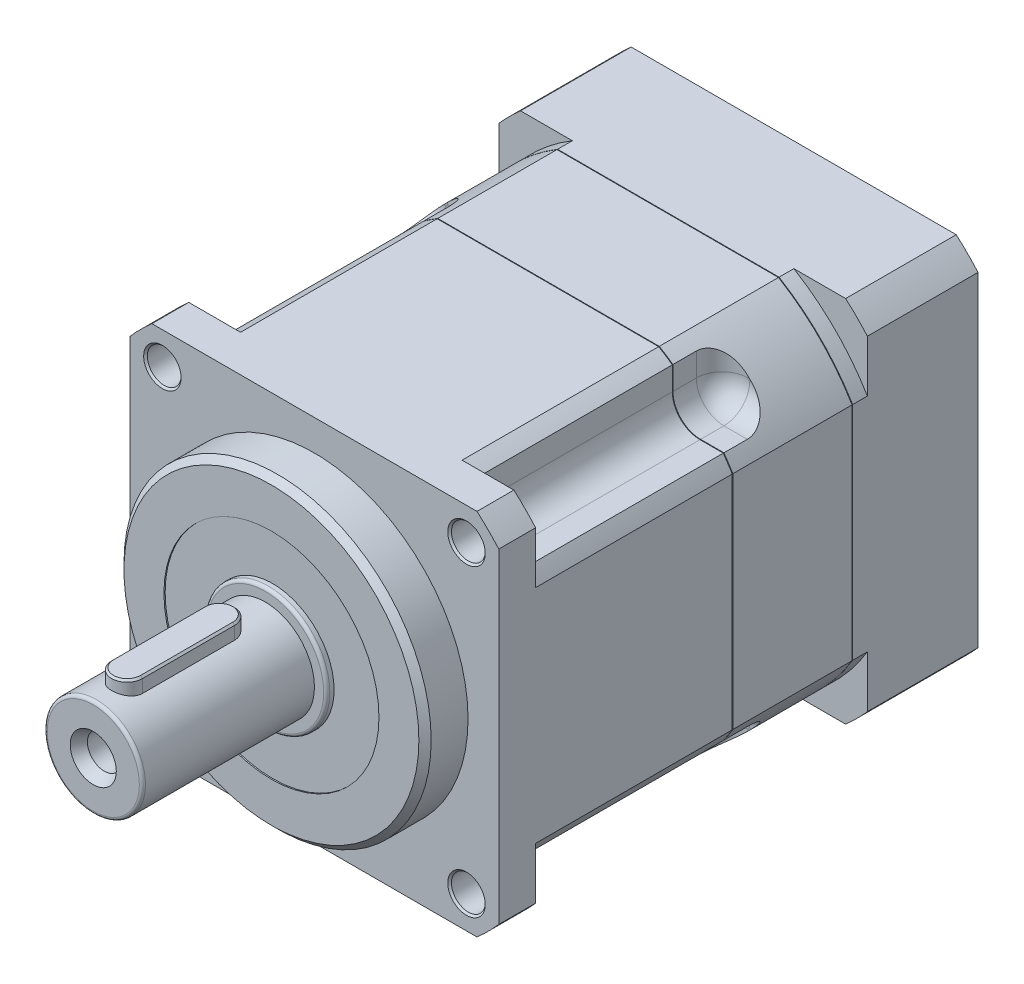
from build123d import *

# Parameters (mm, degrees)
EXTRUDE_1_DEPTH          = 6
SKETCH_2_R               = 25
EXTRUDE_2_DEPTH          = 7
EXTRUDE_3_DEPTH          = 32
SKETCH_4_W               = 13.908632067
SKETCH_4_H               = 13.141259263
CUT_EXTRUDE_1_DEPTH      = 32
PATTERN_CIRCULAR_1_COUNT = 4
FILLET_1_R               = 4.5
SKETCH_5_R               = 2.75
CUT_EXTRUDE_2_DEPTH      = 32
PATTERN_CIRCULAR_2_COUNT = 4
EXTRUDE_4_DEPTH          = 19.4
SKETCH_7_W               = 15.922985677
SKETCH_7_H               = 14.292318469
CUT_EXTRUDE_3_DEPTH      = 8
PATTERN_CIRCULAR_3_COUNT = 4
FILLET_2_R               = 4.5
FILLET_3_R               = 4.2
CHAMFER_1_SIZE           = 1
EXTRUDE_5_DEPTH          = 2.4
EXTRUDE_START            = 18
EXTRUDE_6_DEPTH          = 18
SKETCH_10_R              = 25
CUT_EXTRUDE_4_DEPTH      = 5
SKETCH_11_R              = 4
CUT_EXTRUDE_5_DEPTH      = 12
PATTERN_CIRCULAR_4_COUNT = 4
SKETCH_12_R              = 4
CUT_EXTRUDE_6_DEPTH      = 12
PATTERN_CIRCULAR_5_COUNT = 2
SKETCH_13_R              = 19
CUT_EXTRUDE_7_DEPTH      = 13
SKETCH_14_R              = 3
EXTRUDE_7_DEPTH          = 6
PATTERN_CIRCULAR_6_COUNT = 4
SKETCH_15_R              = 3
EXTRUDE_8_DEPTH          = 6
PATTERN_CIRCULAR_7_COUNT = 2
PATTERN_CIRCULAR_8_COUNT = 4
SKETCH_18_R              = 16.5
EXTRUDE_9_DEPTH          = 11.5
CHAMFER_2_SIZE           = 1
SKETCH_19_R              = 7
CUT_EXTRUDE_8_DEPTH      = 34
SKETCH_20_W              = 35.682835372
SKETCH_20_H              = 1
CUT_EXTRUDE_9_DEPTH      = 11.5
SKETCH_21_R              = 8
EXTRUDE_10_DEPTH         = 29
SKETCH_22_R              = 10
EXTRUDE_11_DEPTH         = 1
FILLET_4_R               = 0.5
FILLET_5_R               = 0.5
CUT_EXTRUDE_START        = -0.2
SKETCH_23_R              = 17.5
SKETCH_23_R_2            = 10
CUT_EXTRUDE_10_DEPTH     = 0.2
EXTRUDE_12_DEPTH         = 10
CHAMFER_3_SIZE           = 0.3
SKETCH_25_R              = 2.75
CUT_EXTRUDE_11_DEPTH     = 4.8
SKETCH_26_R              = 3.75
SKETCH_27_R              = 2.75


with BuildPart() as part:
    # 草图1 → 凸台-拉伸1 (new body)
    with BuildSketch(Plane.XY):
        with BuildLine():
            Line((-26.457513111, 30), (26.457513111, 30))
            ThreePointArc((26.457513111, 30), (28.284271247, 28.284271247), (30, 26.457513111))
            Line((30, 26.457513111), (30, -26.457513111))
            ThreePointArc((30, -26.457513111), (28.284271247, -28.284271247), (26.457513111, -30))
            Line((26.457513111, -30), (-26.457513111, -30))
            ThreePointArc((-26.457513111, -30), (-28.284271247, -28.284271247), (-30, -26.457513111))
            Line((-30, -26.457513111), (-30, 26.457513111))
            ThreePointArc((-30, 26.457513111), (-28.284271247, 28.284271247), (-26.457513111, 30))
        make_face()
    extrude(amount=EXTRUDE_1_DEPTH)

    # 草图2 → 凸台-拉伸2 (add)
    with BuildSketch(Plane.XY.offset(6)):
        Circle(SKETCH_2_R)
    extrude(amount=EXTRUDE_2_DEPTH)

    # 草图3 → 凸台-拉伸3 (add)
    with BuildSketch(Plane(origin=(0, 0, 0), x_dir=(-1, 0, 0), z_dir=(0, 0, -1))):
        with BuildLine():
            Line((-18.027756377, 30), (18.027756377, 30))
            ThreePointArc((18.027756377, 30), (24.748737342, 24.748737342), (30, 18.027756377))
            Line((30, 18.027756377), (30, -18.027756377))
            ThreePointArc((30, -18.027756377), (24.748737342, -24.748737342), (18.027756377, -30))
            Line((18.027756377, -30), (-18.027756377, -30))
            ThreePointArc((-18.027756377, -30), (-24.748737342, -24.748737342), (-30, -18.027756377))
            Line((-30, -18.027756377), (-30, 18.027756377))
            ThreePointArc((-30, 18.027756377), (-24.748737342, 24.748737342), (-18.027756377, 30))
        make_face()
    extrude(amount=EXTRUDE_3_DEPTH)

    # 草图4 → 切除-拉伸1 (cut)
    with BuildSketch(Plane(origin=(0, 0, -32), x_dir=(-1, 0, 0), z_dir=(0, 0, -1))):
        with Locations((-27.204316033, 26.820629632)):
            Rectangle(SKETCH_4_W, SKETCH_4_H)
    cut_extrude_1 = extrude(amount=-CUT_EXTRUDE_1_DEPTH, mode=Mode.SUBTRACT)

    # 阵列(圆周)1: 切除-拉伸1 ×4 about axis
    pattern_circular_1_axis = Axis((0, 0, 0), (0, 0, 1))
    for i in range(1, PATTERN_CIRCULAR_1_COUNT):
        add(cut_extrude_1.rotate(pattern_circular_1_axis, i * 360 / PATTERN_CIRCULAR_1_COUNT), mode=Mode.SUBTRACT)

    # 圆角1
    fillet_1_edges = [part.edges().sort_by_distance(p)[0] for p in [
        (-20.25, -20.25, -16),
        (20.25, -20.25, -16),
        (20.25, 20.25, -16),
        (-20.25, 20.25, -16),
    ]]
    fillet(fillet_1_edges, radius=FILLET_1_R)

    # 草图5 → 切除-拉伸2 (cut)
    with BuildSketch(Plane.XY.offset(6)):
        with Locations((-24.748737342, 24.748737342)):
            Circle(SKETCH_5_R)
    cut_extrude_2 = extrude(amount=-CUT_EXTRUDE_2_DEPTH, mode=Mode.SUBTRACT)

    # 阵列(圆周)2: 切除-拉伸2 ×4 about axis
    pattern_circular_2_axis = Axis((0, 0, 0), (0, 0, 1))
    for i in range(1, PATTERN_CIRCULAR_2_COUNT):
        add(cut_extrude_2.rotate(pattern_circular_2_axis, i * 360 / PATTERN_CIRCULAR_2_COUNT), mode=Mode.SUBTRACT)

    # 倒角1
    chamfer_1_edges = [part.edges().sort_by_distance(p)[0] for p in [
        (-25, 0, 13),
    ]]
    chamfer(chamfer_1_edges, length=CHAMFER_1_SIZE)

    # 草图21 → 凸台-拉伸10 (add)
    with BuildSketch(Plane.XY.offset(13)):
        with Locations(Location((0, 0, 0), (0, 0, 180))):
            Circle(SKETCH_21_R)
    extrude(amount=EXTRUDE_10_DEPTH)

    # 草图22 → 凸台-拉伸11 (add)
    with BuildSketch(Plane.XY.offset(13)):
        Circle(SKETCH_22_R)
    extrude(amount=EXTRUDE_11_DEPTH)

    # 圆角4
    fillet_4_edges = [part.edges().sort_by_distance(p)[0] for p in [
        (-10, 0, 14),
    ]]
    fillet(fillet_4_edges, radius=FILLET_4_R)

    # 圆角5
    fillet_5_edges = [part.edges().sort_by_distance(p)[0] for p in [
        (8, 0, 42),
    ]]
    fillet(fillet_5_edges, radius=FILLET_5_R)

    # 草图23 → 切除-拉伸10 (cut)
    with BuildSketch(Plane.XY.offset(13).offset(CUT_EXTRUDE_START)):
        Circle(SKETCH_23_R)
        Circle(SKETCH_23_R_2, mode=Mode.SUBTRACT)
    extrude(amount=CUT_EXTRUDE_10_DEPTH, mode=Mode.SUBTRACT)

    # 草图24 → 凸台-拉伸12 (add)
    with BuildSketch(Plane(origin=(0, 0, 0), x_dir=(1, 0, 0), z_dir=(0, 1, 0))):
        with BuildLine():
            Line((-2.5, -21.5), (-2.5, -36.5))
            ThreePointArc((-2.5, -36.5), (0, -39), (2.5, -36.5))
            Line((2.5, -36.5), (2.5, -21.5))
            ThreePointArc((2.5, -21.5), (0, -19), (-2.5, -21.5))
        make_face()
    extrude(amount=EXTRUDE_12_DEPTH)

    # 倒角3
    chamfer_3_edges = [part.edges().sort_by_distance(p)[0] for p in [
        (-27.498737342, 24.748737342, 6),
        (24.748737342, 27.498737342, 6),
        (27.498737342, -24.748737342, 6),
        (-24.748737342, -27.498737342, 6),
        (0, 10, 19),
        (-2.5, 10, 29),
        (0, 10, 39),
        (2.5, 10, 29),
    ]]
    chamfer(chamfer_3_edges, length=CHAMFER_3_SIZE)

    # 草图25 → 切除-拉伸11 (cut)
    with BuildSketch(Plane.XY.offset(42)):
        Circle(SKETCH_25_R)
    extrude(amount=-CUT_EXTRUDE_11_DEPTH, mode=Mode.SUBTRACT)

    # 草图26 → 切除-放样1 section 0
    with BuildSketch(Plane.XY.offset(42)):
        Circle(SKETCH_26_R)
    # 草图27 → 切除-放样1 section 1
    with BuildSketch(Plane.XY.offset(40.2)):
        Circle(SKETCH_27_R)
    loft(mode=Mode.SUBTRACT)

    # 草图28 → M5 螺纹孔1 (revolve, cut)
    with BuildSketch(Plane(origin=(0, 0, 37.2), x_dir=(0, -1, 0), z_dir=(1, 0, 0))):
        Polygon((0, 0), (0, 20.4618073), (2.1, 19.2), (2.1, 0), align=None)
    revolve(axis=Axis((0, 0, 43.55), (0, 0, -1)), mode=Mode.SUBTRACT)


with BuildPart() as body_2:
    # 草图6 → 凸台-拉伸4 (new body)
    with BuildSketch(Plane(origin=(0, 0, -32.1), x_dir=(-1, 0, 0), z_dir=(0, 0, -1))):
        with BuildLine():
            Line((-18.027756377, 30), (18.027756377, 30))
            ThreePointArc((18.027756377, 30), (24.748737342, 24.748737342), (30, 18.027756377))
            Line((30, 18.027756377), (30, -18.027756377))
            ThreePointArc((30, -18.027756377), (24.748737342, -24.748737342), (18.027756377, -30))
            Line((18.027756377, -30), (-18.027756377, -30))
            ThreePointArc((-18.027756377, -30), (-24.748737342, -24.748737342), (-30, -18.027756377))
            Line((-30, -18.027756377), (-30, 18.027756377))
            ThreePointArc((-30, 18.027756377), (-24.748737342, 24.748737342), (-18.027756377, 30))
        make_face()
    extrude(amount=EXTRUDE_4_DEPTH)

    # 草图7 → 切除-拉伸3 (cut)
    with BuildSketch(Plane.XY.offset(-32.1)):
        with Locations((-28.211492838, 27.396159235)):
            Rectangle(SKETCH_7_W, SKETCH_7_H)
    cut_extrude_3 = extrude(amount=-CUT_EXTRUDE_3_DEPTH, mode=Mode.SUBTRACT)

    # 阵列(圆周)3: 切除-拉伸3 ×4 about axis
    pattern_circular_3_axis = Axis((0, 0, 0), (0, 0, 1))
    for i in range(1, PATTERN_CIRCULAR_3_COUNT):
        add(cut_extrude_3.rotate(pattern_circular_3_axis, i * 360 / PATTERN_CIRCULAR_3_COUNT), mode=Mode.SUBTRACT)

    # 圆角2
    fillet_2_edges = [body_2.edges().sort_by_distance(p)[0] for p in [
        (-20.25, 20.25, -36.1),
        (-20.25, -20.25, -36.1),
        (20.25, -20.25, -36.1),
        (20.25, 20.25, -36.1),
    ]]
    fillet(fillet_2_edges, radius=FILLET_2_R)

    # 圆角3
    fillet_3_edges = [body_2.edges().sort_by_distance(p)[0] for p in [
        (21.568019485, 21.568019485, -40.1),
        (-20.25, 26.648555093, -40.1),
        (-21.568019485, 21.568019485, -40.1),
        (-26.648555093, 20.25, -40.1),
        (-20.25, -26.648555093, -40.1),
        (26.648555093, -20.25, -40.1),
        (20.25, 26.648555093, -40.1),
        (-26.648555093, -20.25, -40.1),
        (-21.568019485, -21.568019485, -40.1),
        (20.25, -26.648555093, -40.1),
        (21.568019485, -21.568019485, -40.1),
        (26.648555093, 20.25, -40.1),
    ]]
    fillet(fillet_3_edges, radius=FILLET_3_R)


with BuildPart() as body_3:
    # 草图8 → 凸台-拉伸5 (new body)
    with BuildSketch(Plane(origin=(0, 0, -51.6), x_dir=(-1, 0, 0), z_dir=(0, 0, -1))):
        with BuildLine():
            Line((18.027756377, 30), (-18.027756377, 30))
            ThreePointArc((-18.027756377, 30), (-24.748737342, 24.748737342), (-30, 18.027756377))
            Line((-30, 18.027756377), (-30, -18.027756377))
            ThreePointArc((-30, -18.027756377), (-24.748737342, -24.748737342), (-18.027756377, -30))
            Line((-18.027756377, -30), (18.027756377, -30))
            ThreePointArc((18.027756377, -30), (24.748737342, -24.748737342), (30, -18.027756377))
            Line((30, -18.027756377), (30, 18.027756377))
            ThreePointArc((30, 18.027756377), (24.748737342, 24.748737342), (18.027756377, 30))
        make_face()
    extrude(amount=EXTRUDE_5_DEPTH)

    # 草图9 → 凸台-拉伸6 (add)
    with BuildSketch(Plane(origin=(0, 0, -54), x_dir=(-1, 0, 0), z_dir=(0, 0, -1)).offset(EXTRUDE_START)):
        with BuildLine():
            Line((-26.457513111, 30), (26.457513111, 30))
            ThreePointArc((26.457513111, 30), (28.284271247, 28.284271247), (30, 26.457513111))
            Line((30, 26.457513111), (30, -26.457513111))
            ThreePointArc((30, -26.457513111), (28.284271247, -28.284271247), (26.457513111, -30))
            Line((26.457513111, -30), (-26.457513111, -30))
            ThreePointArc((-26.457513111, -30), (-28.284271247, -28.284271247), (-30, -26.457513111))
            Line((-30, -26.457513111), (-30, 26.457513111))
            ThreePointArc((-30, 26.457513111), (-28.284271247, 28.284271247), (-26.457513111, 30))
        make_face()
    extrude(amount=-EXTRUDE_6_DEPTH)

    # 草图10 → 切除-拉伸4 (cut)
    with BuildSketch(Plane(origin=(0, 0, -72), x_dir=(-1, 0, 0), z_dir=(0, 0, -1))):
        Circle(SKETCH_10_R)
    extrude(amount=-CUT_EXTRUDE_4_DEPTH, mode=Mode.SUBTRACT)

    # 草图11 → 切除-拉伸5 (cut)
    with BuildSketch(Plane(origin=(0, 0, -72), x_dir=(-1, 0, 0), z_dir=(0, 0, -1))):
        with Locations((6.470476128, -24.148145657)):
            Circle(SKETCH_11_R)
    cut_extrude_5 = extrude(amount=-CUT_EXTRUDE_5_DEPTH, mode=Mode.SUBTRACT)

    # 阵列(圆周)4: 切除-拉伸5 ×4 about axis
    pattern_circular_4_axis = Axis((0, 0, 0), (0, 0, 1))
    for i in range(1, PATTERN_CIRCULAR_4_COUNT):
        add(cut_extrude_5.rotate(pattern_circular_4_axis, i * 360 / PATTERN_CIRCULAR_4_COUNT), mode=Mode.SUBTRACT)

    # 草图12 → 切除-拉伸6 (cut)
    with BuildSketch(Plane(origin=(0, 0, -72), x_dir=(-1, 0, 0), z_dir=(0, 0, -1))):
        with Locations((-15.733009776, -19.428649036)):
            Circle(SKETCH_12_R)
    cut_extrude_6 = extrude(amount=-CUT_EXTRUDE_6_DEPTH, mode=Mode.SUBTRACT)

    # 阵列(圆周)5: 切除-拉伸6 ×2 about axis
    pattern_circular_5_axis = Axis((0, 0, 0), (0, 0, 1))
    for i in range(1, PATTERN_CIRCULAR_5_COUNT):
        add(cut_extrude_6.rotate(pattern_circular_5_axis, i * 360 / PATTERN_CIRCULAR_5_COUNT), mode=Mode.SUBTRACT)

    # 草图13 → 切除-拉伸7 (cut)
    with BuildSketch(Plane(origin=(0, 0, -67), x_dir=(-1, 0, 0), z_dir=(0, 0, -1))):
        Circle(SKETCH_13_R)
    extrude(amount=-CUT_EXTRUDE_7_DEPTH, mode=Mode.SUBTRACT)

    # 草图14 → 凸台-拉伸7 (add)
    with BuildSketch(Plane(origin=(0, 0, -60), x_dir=(-1, 0, 0), z_dir=(0, 0, -1))):
        with Locations((-6.470476128, 24.148145657)):
            Circle(SKETCH_14_R)
        Polygon((-5.6436782, 25.788974755), (-7.478076846, 25.684588215), (-8.304874774, 24.043759117), (-7.297274055, 22.507316559), (-5.462875409, 22.611703099), (-4.636077481, 24.252532197), align=None, mode=Mode.SUBTRACT)
    extrude_7 = extrude(amount=EXTRUDE_7_DEPTH)

    # 阵列(圆周)6: 凸台-拉伸7 ×4 about axis
    pattern_circular_6_axis = Axis((0, 0, 0), (0, 0, 1))
    for i in range(1, PATTERN_CIRCULAR_6_COUNT):
        add(extrude_7.rotate(pattern_circular_6_axis, i * 360 / PATTERN_CIRCULAR_6_COUNT))

    # 草图15 → 凸台-拉伸8 (add)
    with BuildSketch(Plane(origin=(0, 0, -60), x_dir=(-1, 0, 0), z_dir=(0, 0, -1))):
        with Locations((-15.733009776, -19.428649036)):
            Circle(SKETCH_15_R)
        Polygon((-14.815671669, -17.876419751), (-16.618610716, -17.858096289), (-17.535948824, -19.410325574), (-16.650347884, -20.980878322), (-14.847408836, -20.999201784), (-13.930070729, -19.446972499), align=None, mode=Mode.SUBTRACT)
    extrude_8 = extrude(amount=EXTRUDE_8_DEPTH)

    # 阵列(圆周)7: 凸台-拉伸8 ×2 about axis
    pattern_circular_7_axis = Axis((0, 0, 0), (0, 0, 1))
    for i in range(1, PATTERN_CIRCULAR_7_COUNT):
        add(extrude_8.rotate(pattern_circular_7_axis, i * 360 / PATTERN_CIRCULAR_7_COUNT))

    # 草图17 → M4 螺纹孔1 (revolve, cut)
    with BuildSketch(Plane(origin=(24.748737342, 24.748737342, -72), x_dir=(0, 1, 0), z_dir=(1, 0, 0))):
        Polygon((0, 0), (0, 16.491420021), (1.65, 15.5), (1.65, 0), align=None)
    hole_wizard_m4_1 = revolve(axis=Axis((24.748737342, 24.748737342, -78.35), (0, 0, 1)), mode=Mode.SUBTRACT)

    # 阵列(圆周)8: M4 螺纹孔1 ×4 about axis
    pattern_circular_8_axis = Axis((0, 0, 0), (0, 0, 1))
    for i in range(1, PATTERN_CIRCULAR_8_COUNT):
        add(hole_wizard_m4_1.rotate(pattern_circular_8_axis, i * 360 / PATTERN_CIRCULAR_8_COUNT), mode=Mode.SUBTRACT)

    # 草图18 → 凸台-拉伸9 (add)
    with BuildSketch(Plane(origin=(0, 0, -54), x_dir=(-1, 0, 0), z_dir=(0, 0, -1))):
        Circle(SKETCH_18_R)
    extrude(amount=EXTRUDE_9_DEPTH)

    # 倒角2
    chamfer_2_edges = [body_3.edges().sort_by_distance(p)[0] for p in [
        (16.5, 0, -65.5),
    ]]
    chamfer(chamfer_2_edges, length=CHAMFER_2_SIZE)


with BuildPart() as cut_extrude_8_tool:
    # 草图19 → 切除-拉伸8 (new body)
    with BuildSketch(Plane(origin=(0, 0, -72), x_dir=(-1, 0, 0), z_dir=(0, 0, -1))):
        Circle(SKETCH_19_R)
    extrude(amount=-CUT_EXTRUDE_8_DEPTH)


with BuildPart() as body_2_1:
    add(body_2.part)

    # 切除-拉伸8: cut by cut_extrude_8_tool
    add(cut_extrude_8_tool.part, mode=Mode.SUBTRACT)


with BuildPart() as body_3_1:
    add(body_3.part)

    # 切除-拉伸8: cut by cut_extrude_8_tool
    add(cut_extrude_8_tool.part, mode=Mode.SUBTRACT)

    # 草图20 → 切除-拉伸9 (cut)
    with BuildSketch(Plane(origin=(0, 0, -65.5), x_dir=(-1, 0, 0), z_dir=(0, 0, -1))):
        with Locations((0.383686402, 0)):
            Rectangle(SKETCH_20_W, SKETCH_20_H)
    extrude(amount=-CUT_EXTRUDE_9_DEPTH, mode=Mode.SUBTRACT)


solid = Compound([part.part, body_2_1.part, body_3_1.part])
